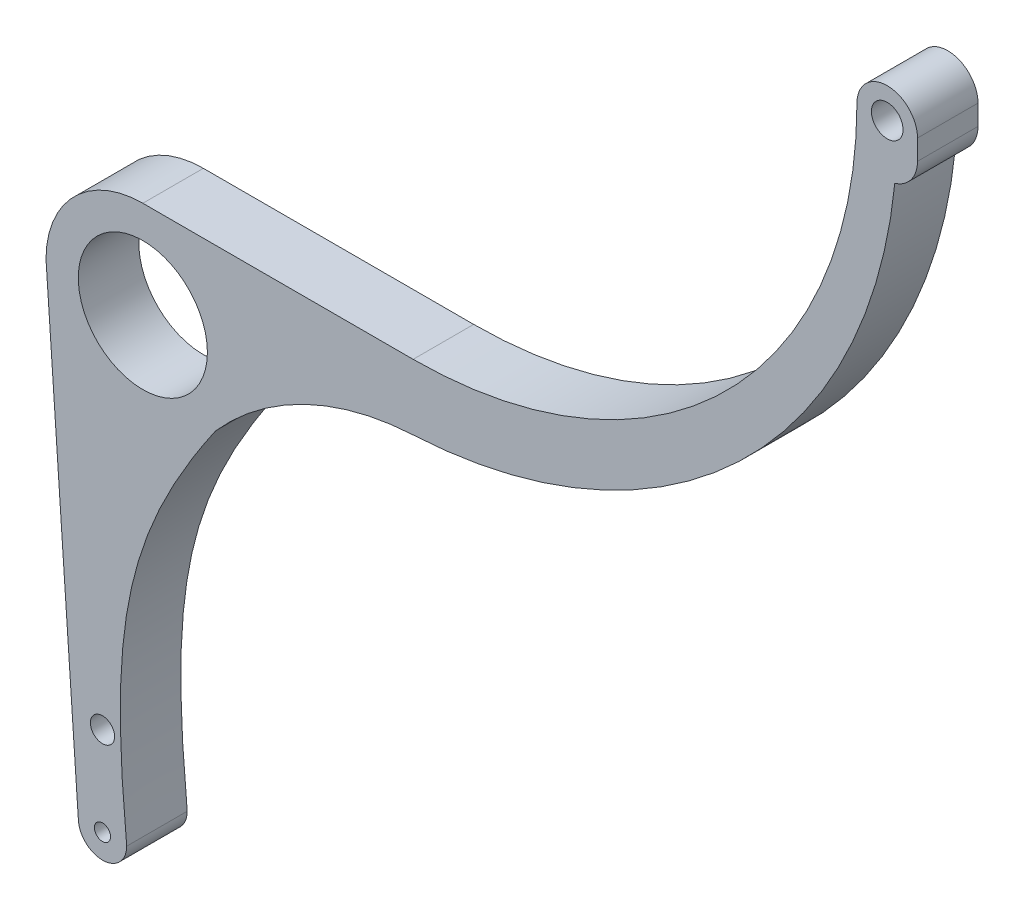
SolidWorks part; units mm, degrees
ref_plane "前视基准面" through (0, 0, 0) normal (0, 0, 1) x (1, 0, 0)
ref_plane "上视基准面" through (0, 0, 0) normal (0, 1, 0) x (1, 0, 0)
ref_plane "右视基准面" through (0, 0, 0) normal (1, 0, 0) x (0, 0, -1)
other "Configuration Table"
sketch "草图1" plane through (0, 0, 0) normal (0, 0, 1) x (1, 0, 0)
  line L0 (-60.8711, 0) -> (72.3657, 0) construction
  line L1 (-84.052, 116) -> (106.5467, 116) construction
  line L2 (0, 22) -> (0, -18.0859) construction
  line L3 (0, -18.0859) -> (10, -18.0859) construction
  line L4 (10, -18.0859) -> (10, 407.7959) construction
  line L5 (-9, 59.8208) -> (-9, -18.0859) construction
  line L6 (-14, 116) -> (-6, 0)
  line L7 (-176.4012, 250) -> (270.3663, 250) construction
  line L8 (77, 485.9134) -> (77, 110.3328) construction
  line L9 (10, 140) -> (77, 140)
  line L10 (187, 250) -> (194.5, 250) construction
  line L11 (202, 250) -> (202, 245)
  line L12 (202, 245) -> (194.1788, 245) construction
  line L13 (70.6056, 267.7759) -> (70.6056, 254.1409) construction
  line L14 (4.2515, 53.8248) -> (157.9856, 53.8248) construction
  line L15 (80.543, 130.5208) -> (80.543, 47.5555) construction
  line L16 (4.7446, 100.1309) -> (49.2871, 100.1309) construction
  line L17 (-29.78, 360) -> (265.8488, 360) construction
  circle A0 centre (0, 0) radius 2
  arc A1 (-6, 0) -> (6, 0) centre (0, 0) ccw
  circle A2 centre (10, 116) radius 16
  arc A3 (10, 140) -> (-14, 116) centre (10, 116) ccw
  circle A4 centre (77, 250) radius 115 construction
  arc A5 (77, 140) -> (187, 250) centre (77, 250) ccw
  arc A6 (202, 250) -> (187, 250) centre (194.5, 250) ccw
  arc A9 (196.3799, 237.4949) -> (202, 245) centre (194.1788, 245) ccw
  arc A10 (77, 123.7674) -> (28.0048, 100.1309) centre (80.543, 53.8248) ccw
  arc A11 (77, 123.7674) -> (196.3799, 237.4949) centre (70.6056, 250) ccw
  circle A12 centre (194.5, 250) radius 3.919
  circle A13 centre (0, 22) radius 3
  spline S0 degree 3 poles (6, 0) (1.5887, 45.6809) (5.6041, 67.6432) (28.0048, 100.1309) knots 0 0 0 0 0.788155 0.788155 0.788155 0.788155
  dimension "D1" = 4
  dimension "D2" = 12
  dimension "D5" = 19
  dimension "D6" = 134
  dimension "D8" = 230
  dimension "D9" = 6.3944
  dimension "D10" = 62.1752
  dimension "D12" = 15.8691
  dimension "D14" = 24
  dimension "D15" = 6
  dimension "D16" = 7.838
  dimension "D17" = 7.5
  dimension "D18" = 220
  dimension "D3" = 116
  dimension "D4" = 9
  dimension "D7" = 67
  dimension "D11" = 70.543
  dimension "D13" = 22
sketch "草图3" plane through (0, 0, 0) normal (0, 0, 1) x (1, 0, 0)
extrude "凸台-拉伸3" add sketch "草图1" along normal blind 15
